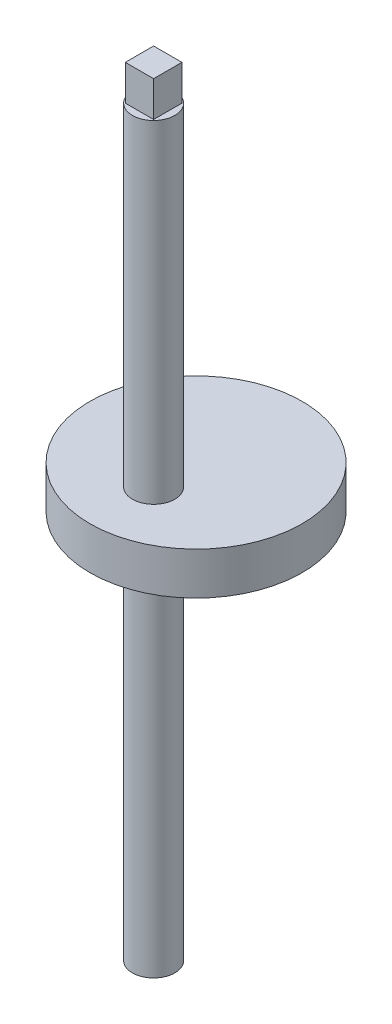
from build123d import *

# Parameters (mm, degrees)
SKETCH1_R           = 15
BOSS_EXTRUDE1_DEPTH = 3
SKETCH3_R           = 3
BOSS_EXTRUDE2_DEPTH = 55
SKETCH4_R           = 3
SKETCH4_W           = 4
SKETCH4_H           = 4
CUT_EXTRUDE1_DEPTH  = 5


with BuildPart() as part:
    # Sketch1 → Boss-Extrude1 (new, symmetric)
    with BuildSketch(Plane(origin=(0, 0, 0), x_dir=(1, 0, 0), z_dir=(0, 1, 0))):
        with Locations(Location((0, 0, 0), (0, 0, 270))):
            Circle(SKETCH1_R)
    extrude(amount=BOSS_EXTRUDE1_DEPTH, both=True)

    # Sketch3 → Boss-Extrude2 (add, symmetric)
    with BuildSketch(Plane(origin=(0, 0, 0), x_dir=(1, 0, 0), z_dir=(0, 1, 0))):
        with Locations(Location((0, -6, 0), (0, 0, 270))):
            Circle(SKETCH3_R)
    extrude(amount=BOSS_EXTRUDE2_DEPTH, both=True)

    # Sketch4 → Cut-Extrude1 (cut)
    with BuildSketch(Plane(origin=(0, 55, 0), x_dir=(1, 0, 0), z_dir=(0, 1, 0))):
        with Locations(Location((0, -6, 0), (0, 0, 270))):
            Circle(SKETCH4_R)
        with Locations((0, -6)):
            Rectangle(SKETCH4_W, SKETCH4_H, mode=Mode.SUBTRACT)
    extrude(amount=-CUT_EXTRUDE1_DEPTH, mode=Mode.SUBTRACT)


solid = part.part
